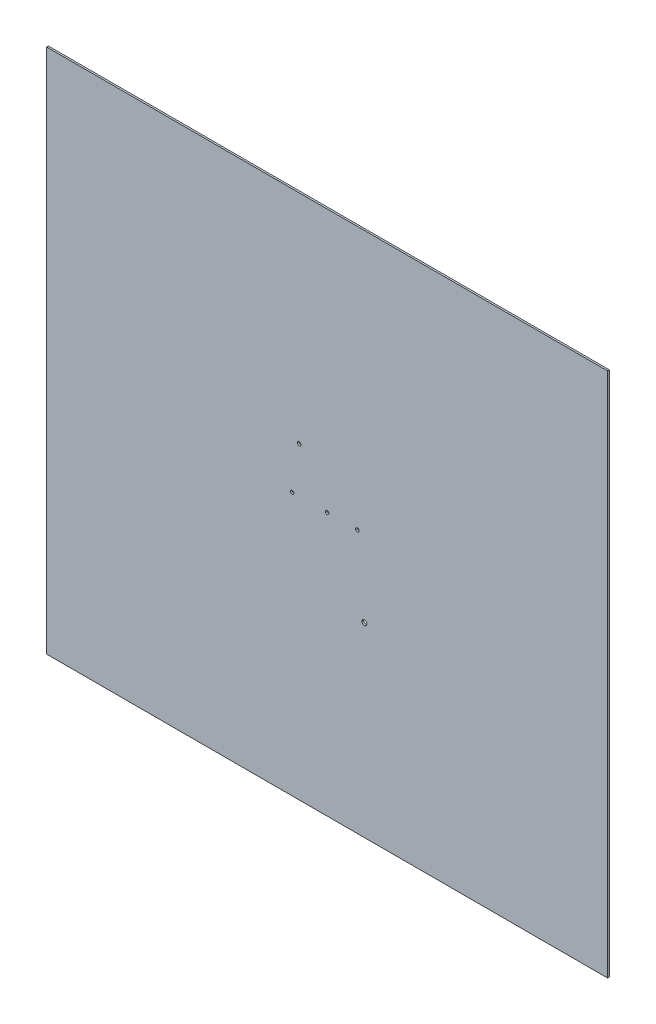
from build123d import *

# Parameters (mm, degrees)
SKETCH1_W           = 1600
SKETCH1_H           = 1500
SKETCH1_R           = 5
SKETCH1_R_2         = 6.865468099
SKETCH1_R_3         = 5.007080458
BOSS_EXTRUDE1_DEPTH = 5


with BuildPart() as part:
    # Sketch1 → Boss-Extrude1 (new body)
    with BuildSketch(Plane.XY):
        Rectangle(SKETCH1_W, SKETCH1_H)
        Circle(SKETCH1_R, mode=Mode.SUBTRACT)
        with Locations((-99.75, 0)):
            Circle(SKETCH1_R, mode=Mode.SUBTRACT)
        with Locations((86.25, 0)):
            Circle(SKETCH1_R, mode=Mode.SUBTRACT)
        with Locations((106.25, -219.089023002)):
            Circle(SKETCH1_R_2, mode=Mode.SUBTRACT)
        with Locations((-79.75, 130)):
            Circle(SKETCH1_R_3, mode=Mode.SUBTRACT)
    extrude(amount=BOSS_EXTRUDE1_DEPTH)


solid = part.part
